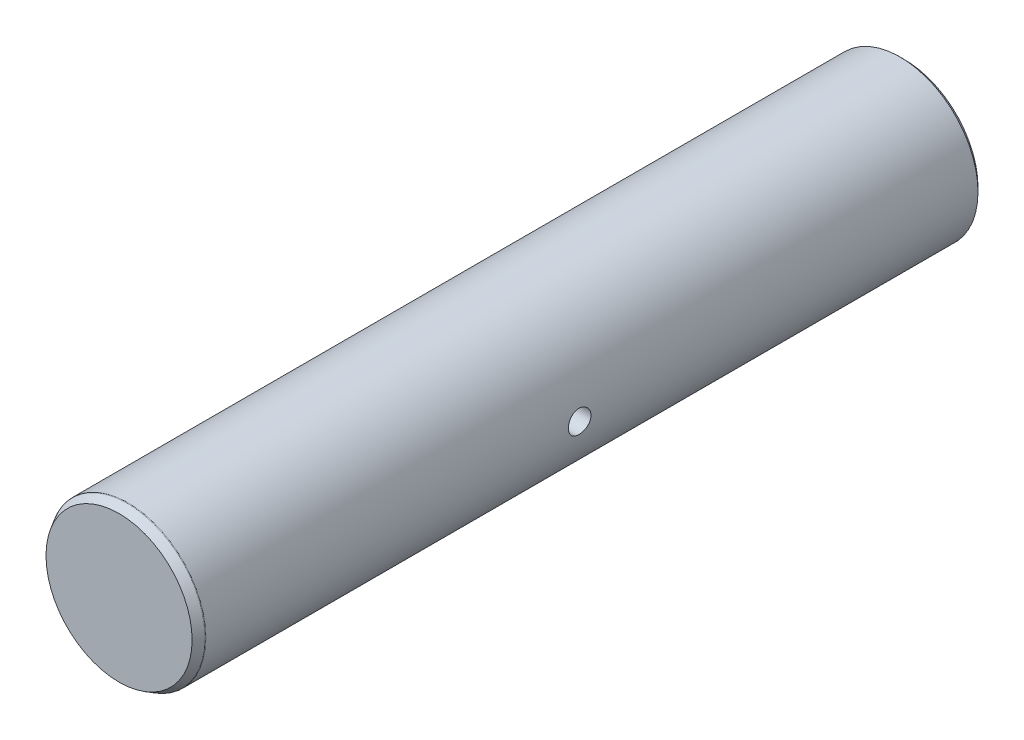
from build123d import *

# Parameters (mm, degrees)
SKETCH_1_R      = 27.5
EXTRUDE_1_DEPTH = 277
MM_1_D          = 6
MM_1_DEPTH      = 10
MM_1_TIP        = 1.802581857
MM_2_D          = 8
MM_2_DEPTH      = 8
MM_2_TIP        = 2.403442476
CHAMFER_1_SIZE  = 1.5
CHAMFER_2_SIZE  = 3
CHAMFER_2_SIZE2 = 1.732050808
FILLET_1_R      = 0.5


with BuildPart() as part:
    # 草图1 → 凸台-拉伸1 (new body)
    with BuildSketch(Plane.XY):
        Circle(SKETCH_1_R)
    extrude(amount=EXTRUDE_1_DEPTH)

    # 大小mm 暗销孔1
    with Locations(Plane(origin=(0, 0, 0), x_dir=(1, 0, 0), z_dir=(0, 0, -1))):
        with Locations((15, 0), (-15, 0)):
            Hole(MM_1_D / 2, depth=MM_1_DEPTH)
            with Locations((0, 0, -(MM_1_DEPTH + MM_1_TIP / 2))):  # 118° drill point
                Cone(0, MM_1_D / 2, MM_1_TIP, mode=Mode.SUBTRACT)

    # 大小mm 暗销孔2
    with Locations(Plane(origin=(27.5, 0, 0), x_dir=(0, 0, -1), z_dir=(1, 0, 0))):
        with Locations((-142, 0)):
            Hole(MM_2_D / 2, depth=MM_2_DEPTH)
            with Locations((0, 0, -(MM_2_DEPTH + MM_2_TIP / 2))):  # 118° drill point
                Cone(0, MM_2_D / 2, MM_2_TIP, mode=Mode.SUBTRACT)

    # 倒角1
    chamfer_1_edges = [part.edges().sort_by_distance(p)[0] for p in [
        (-27.5, 0, 0),
    ]]
    chamfer(chamfer_1_edges, length=CHAMFER_1_SIZE)

    # 倒角2
    chamfer_2_edges = [part.edges().sort_by_distance(p)[0] for p in [
        (-27.5, 0, 277),
    ]]
    chamfer_2_side = [part.faces().sort_by_distance(p)[0] for p in [
        (-27.5, 0, 139.25),
    ]]
    chamfer(chamfer_2_edges, length=CHAMFER_2_SIZE, length2=CHAMFER_2_SIZE2, reference=chamfer_2_side[0])

    # 圆角1
    fillet_1_edges = [part.edges().sort_by_distance(p)[0] for p in [
        (-27.5, 0, 274),
    ]]
    fillet(fillet_1_edges, radius=FILLET_1_R)


solid = part.part
